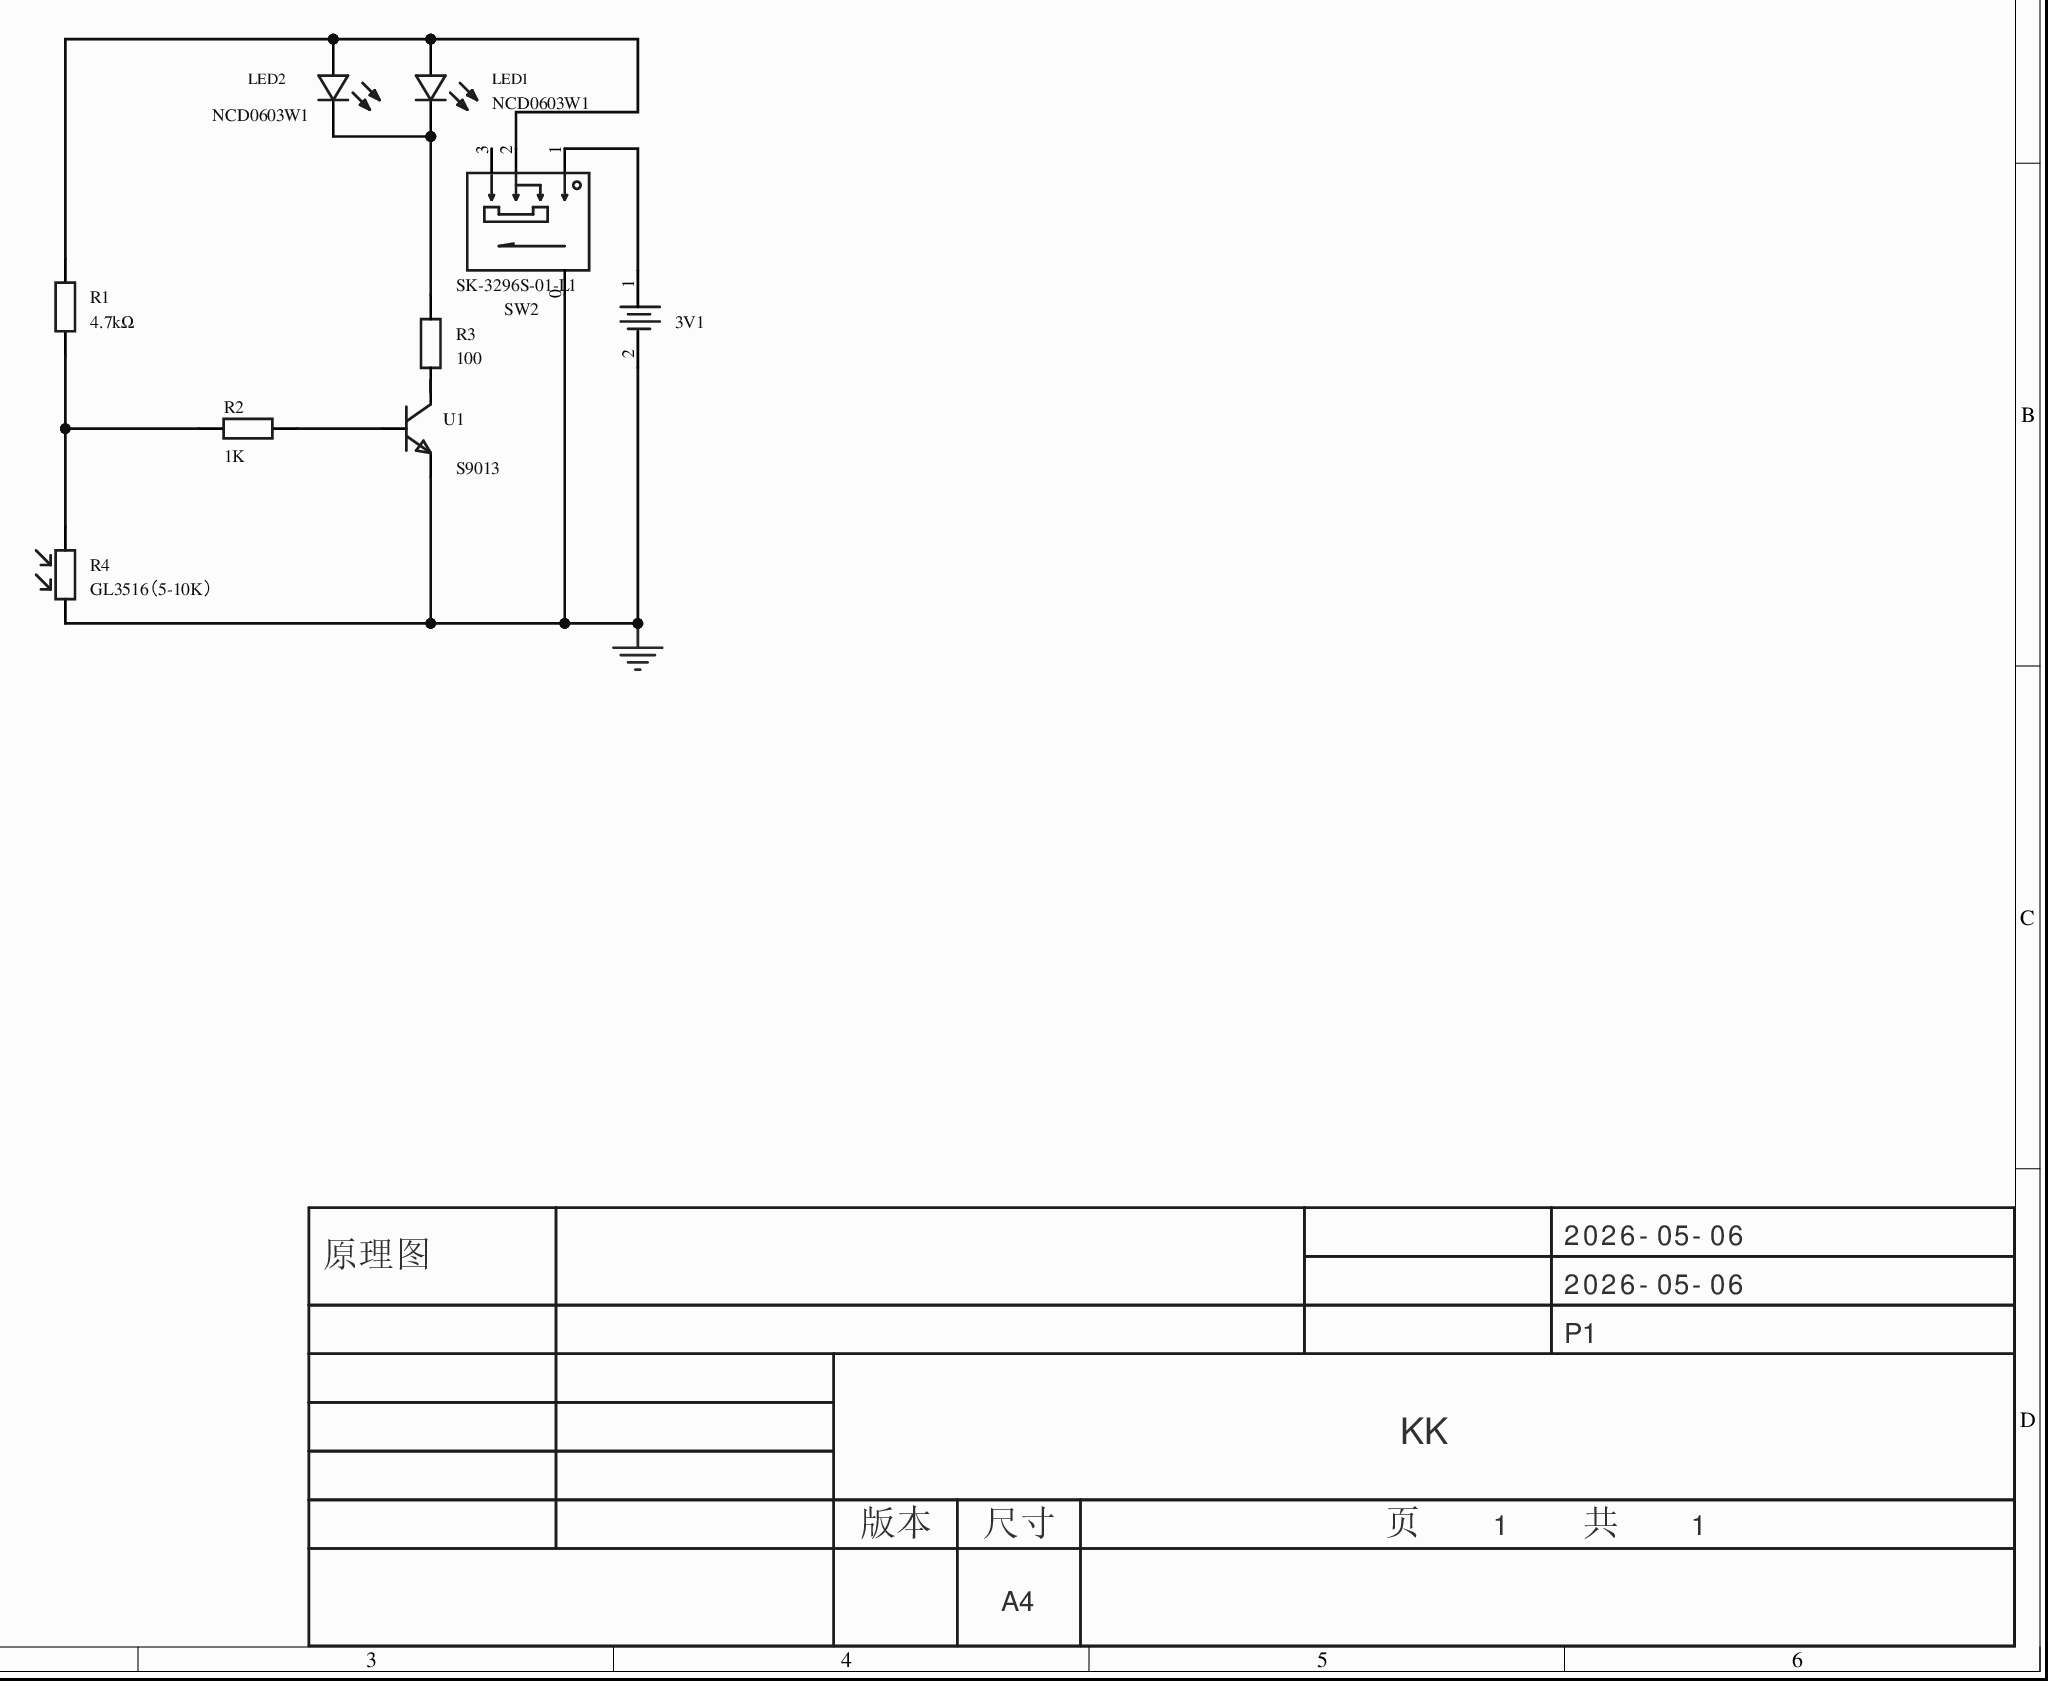
[diagram p0: MISC51059-3.schdoc]
# Altium project MISC51059-2.PrjPcb
1 sheet, 9 parts. Net scope: global (net labels, ports and power ports of the same name join across sheets).
Board file: MISC51059.pcbdoc

## Sheet MISC51059-3.schdoc
size 297 x 209 mm; Version: V1.0; @Project Name: MISC51059; @Update Date: 2026-05-06; @Create Date: 2026-05-06; @Board Name: MISC51059; @Create Time: 21:47:12; @Page Count: 1; @Page No: 1; @Schematic Name: MISC51059; @Update Time: 21:47:12; Size: A4

### Parts
3V1  (no value)  [BAT-TH_CR2032-BS-6-1]
LED1  NCD0603W1  [LED0603-RD]
LED2  NCD0603W1  [LED0603-RD]
R1  4.7kΩ  [R0805]
R2  1K  [R0805]
R3  100  [R0805]
R4  GL3516（5-10K）  [RES-TH_L5.1-W4.3-P3.40-D0.5]
SW2  SK-3296S-01-L1  [SW-SMD_3P-P1.50_L2.7-W6.6]
U1  S9013  [SOT-23-3_L2.9-W1.3-P1.90-LS2.4-BR]

### Nets
GND: 3V1.2 R4.2 SW2.0 U1.2(E)
Net3V1_1: 3V1.1 SW2.1
NetLED1_1: LED1.1(-) LED2.1(-) R3.2
NetLED1_2: LED1.2(+) LED2.2(+) R1.2 SW2.2
NetR1_1: R1.1 R2.2 R4.1
NetR2_1: R2.1 U1.1(B)
NetR3_1: R3.1 U1.3(C)

Not connected (* = marked no-connect by the designer): SW2 3

### Notes on the sheet
- 2026-05-06
- 原理图
- P1
- KK
- 版本
- 尺寸
- A4
- 页    1    共    1

### Library data of the parts
3V1 = CR2032-BS-6-1 COPY: Manufacturer: Q&amp;J; AddInBom: yes; Symbol: CR2032-BS-6-1 COPY; Device: CR2032-BS-6-1 COPY; Supplier: LCSC; Manufacturer Part: CR2032-BS-6-1; Supplier Part: C70377; JLCPCB Part Class: Extended Part; ConvertToPcb: yes; FootprintName: BAT-TH_CR2032-BS-6-1
LED1 LED2 = NCD0603W1: 发光颜色:白灯;; Manufacturer: 国星光电; Symbol: FC-D1608WD-460H5; 3D Model: 1f0d29a91be547639d425604e9b96ebb; 3D Model Transform: 63.7794,32.283,0,0,0,0,0,0,0; Emitted Color: 白灯; AddInBom: yes; Device: NCD0603W1; LCSC Part Name: 白灯 0603白灯   正贴; Supplier Footprint: 0603; Datasheet: https://atta.szlcsc.com/upload/public/pdf/source/20200820/C84265_479E6193713348A548E5CD6D9278BF16.pdf; Supplier: LCSC; Manufacturer Part: NCD0603W1; Supplier Part: C84265; JLCPCB Part Class: 扩展库; ConvertToPcb: yes; FootprintName: LED0603-RD; ModelName: LED0603-RD
R1 R2 = 0805W8F4701T5E: 电阻类型:厚膜电阻;阻值:4.7kΩ;精度:±1%;功率:125mW;温度系数:±100ppm/℃;; Manufacturer: UNI-ROYAL(厚声); 3D Model: 37a81e68749a4138bd2dfa6897b24b85; 3D Model Transform: 78.74,51.181,0,0,0,0,0,-0.0005,0; Tolerance: ±1%; Power(Watts): 125mW; Overload Voltage (Max): 150V; AddInBom: yes; ModelName: R0805_L2.0-W1.3-H0.6; Symbol: 0805W8F4701T5E; Device: 0805W8F4701T5E; LCSC Part Name: 厚膜电阻 4.7kΩ ±1% 125mW; Supplier Footprint: 0805; Datasheet: https://atta.szlcsc.com/upload/public/pdf/source/20200306/C422600_1E6D84923E4A46A82E41ADD87F860B5C.pdf; Type: 厚膜电阻; Temperature Coefficient: ±100ppm/℃; Operating Temperature Range: -55℃~+155℃; Supplier: LCSC; Manufacturer Part: 0805W8F4701T5E; JLCPCB Part Class: 基础库; ConvertToPcb: yes; FootprintName: R0805
  R1: Supplier Part: C17673; Value: 4.7kΩ
  R2: Value: 1K
R3 = Res_0805: Symbol: 电阻; 3D Model: 37a81e68749a4138bd2dfa6897b24b85; 3D Model Transform: 78.74,51.181,0,0,0,0,0,-0.0005,0; ConvertToPcb: yes; ModelName: R0805_L2.0-W1.3-H0.6; Device: Res_0805; Value: 100; Supplier Footprint: 0805; AddInBom: yes; FootprintName: R0805
R4 = GL3516（5-10K）: 光谱峰值(波长):540nm;亮电阻 @ 10Lux:5kΩ~10kΩ;暗电阻:500kΩ;; Manufacturer: JCHL(晶创和立); Symbol: GL3516(5-10K); 3D Model: cb75fcf2d6c94cac811f2579121b8720; 3D Model Transform: 169.291,200.39669,0,0,0,0,-3.937,0,-137.795; Spectral Peak: 540nm; Applied Voltage: 150V; Dark Resistance: 500kΩ; AddInBom: yes; Device: GL3516（5-10K）; LCSC Part Name: 亮电阻:5kΩ~10kΩ 暗电阻:500kΩ; Supplier Footprint: 插件,P=2mm; Datasheet: https://atta.szlcsc.com/upload/public/pdf/source/20130226/1457706594816.pdf; Illuminated Resistance @ 10Lux: 5kΩ~10kΩ; Supplier: LCSC; Manufacturer Part: GL3516（5-10K）; Supplier Part: C11287; JLCPCB Part Class: 扩展库; ConvertToPcb: yes; FootprintName: RES-TH_L5.1-W4.3-P3.40-D0.5; ModelName: RES-TH_L5.1-W4.3-P3.40-D0.5
SW2 = SK-3296S-01-L1: 额定电流(DC):50mA;额定电压(DC):12V;额定电流(AC):50mA;额定电压(AC):12V;电路结构:单刀双掷;安装方式:卧贴;机械寿命:1万次;开关颜色:黑色;; Manufacturer: XKB Connectivity(中国星坤); 3D Model: fac986d38b354d44b3f0357550471109; 3D Model Transform: 307.086,204.724,0,180,0,0,0,-28.898,-19.685; Current Rating (DC): 50mA; Voltage Rating (DC): 12V; Circuit: 单刀双掷; Mechanical Life: 1万次; Actuator Color: 黑色; Actuator Style: 矩形柱状; Pin Style: SMD接片; Switch Length: 7.8mm; Switch Width: 2.75mm; Switch Height: 1.35mm; AddInBom: yes; ModelName: SW-SMD_3P-L6.6-W2.7-LS7.8-P1.50; Symbol: SK-3296S-01-L1; Device: SK-3296S-01-L1; LCSC Part Name: 柄长1.5mm 卧贴双档 滑动开关; Supplier Part: C319020; Manufacturer Part: SK-3296S-01-L1; Supplier Footprint: SMD; JLCPCB Part Class: 扩展库; Datasheet: https://atta.szlcsc.com/upload/public/pdf/source/20211011/33977E7F5E3AE40A3E3DC6795807E20F.pdf; Supplier: LCSC; Current Rating (AC): 50mA; Voltage Rating (AC): 12V; Mounting Style: 卧贴; Operating Temperature: -40℃~+85℃; ConvertToPcb: yes; FootprintName: SW-SMD_3P-P1.50_L2.7-W6.6
U1 = S9013_C5184425: 晶体管类型:NPN;集射极击穿电压(Vceo):25V;集电极电流(Ic):500mA;功率(Pd):300mW;直流电流增益(hFE@Ic,Vce):120@50mA,1V;; Manufacturer: HXY MOSFET(华轩阳电子); 3D Model: c62791f0466c4ae2a892c056b845b0ca; 3D Model Transform: 98.425,114.173,0,180,0,0,0.0005,-0.0005,0; Transistor Type: NPN; Collector-Emitter Breakdown Voltage (Vceo): 25V; Collector Current (Ic): 500mA; Power Dissipation (Pd): 300mW; Collector Cut-Off Current (Icbo): 100nA; Collector-Emitter Saturation Voltage (VCE(sat)@Ic,Ib): 600mV@500mA,50mA; Transition Frequency (fT): 150MHz; AddInBom: yes; ModelName: SOT-23-3P_L2.9-W1.3-H1.0-LS2.4-P0.95; Symbol: S9013_C5184425; Device: S9013_C5184425; LCSC Part Name: NPN 耐压:25V 电流:500mA J3; Supplier Footprint: SOT-23(TO-236); Datasheet: https://atta.szlcsc.com/upload/public/pdf/source/20220926/07971C8172245807F6FC8623E6D5A75D.pdf; DC Current Gain (hFE@Ic,Vce): 120@50mA,1V; Operating Temperature: +150℃; Supplier: LCSC; Supplier Part: C5184425; Manufacturer Part: S9013; JLCPCB Part Class: 扩展库; ConvertToPcb: yes; FootprintName: SOT-23-3_L2.9-W1.3-P1.90-LS2.4-BR